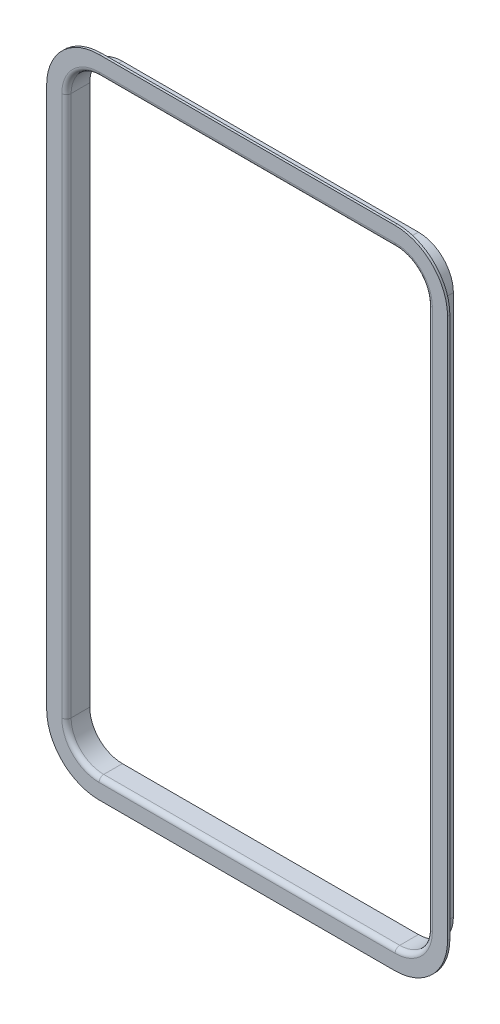
from build123d import *


with BuildPart() as part:
    # Sweep1: sweep along a path in Sketch1
    with BuildLine(Plane.XY) as sweep1_path:
        Line((-127, 260), (127, 260))
        ThreePointArc((127, 260), (146.798989873, 251.798989873), (155, 232))
        Line((155, 232), (155, -232))
        ThreePointArc((155, -232), (146.798989873, -251.798989873), (127, -260))
        Line((127, -260), (-127, -260))
        ThreePointArc((-127, -260), (-146.798989873, -251.798989873), (-155, -232))
        Line((-155, -232), (-155, 232))
        ThreePointArc((-155, 232), (-146.798989873, 251.798989873), (-127, 260))
    # Sketch2 → Sweep1 (sweep)
    with BuildSketch(Plane(origin=(0, 0, 0), x_dir=(1, 0, 0), z_dir=(0, 1, 0))):
        with BuildLine():
            Line((155, 4), (155, 20))
            Line((155, 20), (157, 20))
            Line((157, 20), (157, 4))
            ThreePointArc((157, 4), (157.585786438, 2.585786438), (159, 2))
            Line((159, 2), (172, 2))
            Line((172, 2), (172, 0))
            Line((172, 0), (159, 0))
            ThreePointArc((159, 0), (156.171572875, 1.171572875), (155, 4))
        make_face()
    sweep(path=sweep1_path.line)


solid = part.part
